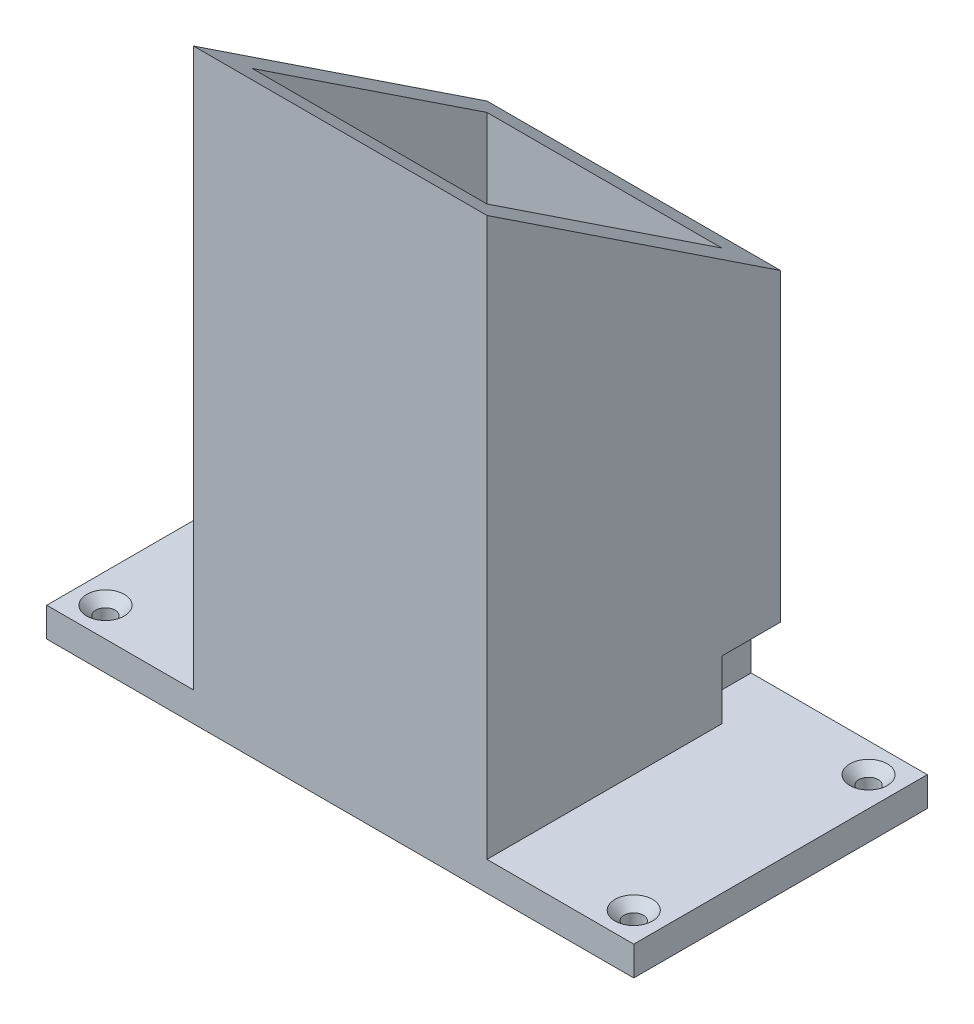
from build123d import *

# Parameters (mm, degrees)
SKETCH1_W                                            = 50
SKETCH1_H                                            = 10
SKETCH1_W_2                                          = 100
SKETCH1_H_2                                          = 200
BOSS_EXTRUDE1_DEPTH                                  = 100
CUT_EXTRUDE1_DEPTH                                   = 174.205080757
CUT_EXTRUDE1_DEPTH_BACK                              = 174.205080757
SKETCH7_W                                            = 80
SKETCH7_H                                            = 80
CUT_EXTRUDE2_DEPTH                                   = 100
SKETCH8_R                                            = 20
CUT_EXTRUDE3_DEPTH                                   = 20
CSK_FOR_M6_HEXAGON_LOBULAR_SOCKET_RAISED_D           = 6.6
CSK_FOR_M6_HEXAGON_LOBULAR_SOCKET_RAISED_CSINK_D     = 12.8
CSK_FOR_M6_HEXAGON_LOBULAR_SOCKET_RAISED_CSINK_ANGLE = 90
SKETCH13_W                                           = 20
SKETCH13_H                                           = 20
CUT_EXTRUDE4_DEPTH                                   = 10


with BuildPart() as part:
    # Sketch1 → Boss-Extrude1 (new body)
    with BuildSketch(Plane.XY):
        with Locations((-75, -95)):
            Rectangle(SKETCH1_W, SKETCH1_H)
        Rectangle(SKETCH1_W_2, SKETCH1_H_2)
        with Locations((75, -95)):
            Rectangle(SKETCH1_W, SKETCH1_H)
    extrude(amount=BOSS_EXTRUDE1_DEPTH)

    # Sketch5 → Cut-Extrude1 (cut, two sides: drawn at the far end of the back side and taken through both)
    with BuildSketch(Plane(origin=(0, 0, 0), x_dir=(0, 0, -1), z_dir=(1, 0, 0)).offset(-CUT_EXTRUDE1_DEPTH_BACK)):
        Polygon((-481.193494813, 352.459484715), (-100, 100), (0, 33.771302986), (381.193494813, -218.688181728), (886.112464242, 543.698807897), (23.725474617, 1114.84647434), align=None)
    extrude(amount=CUT_EXTRUDE1_DEPTH + CUT_EXTRUDE1_DEPTH_BACK, mode=Mode.SUBTRACT)

    # Sketch7 → Cut-Extrude2 (cut, symmetric)
    with BuildSketch(Plane(origin=(0, 0, 0), x_dir=(1, 0, 0), z_dir=(0, 1, 0))):
        with Locations((0, -50)):
            Rectangle(SKETCH7_W, SKETCH7_H)
    extrude(amount=CUT_EXTRUDE2_DEPTH, both=True, mode=Mode.SUBTRACT)

    # Sketch8 → Cut-Extrude3 (cut)
    with BuildSketch(Plane(origin=(0, 0, 0), x_dir=(-1, 0, 0), z_dir=(0, 0, -1))):
        with Locations((0, -40)):
            Circle(SKETCH8_R)
    extrude(amount=-CUT_EXTRUDE3_DEPTH, mode=Mode.SUBTRACT)

    # CSK for M6 Hexagon lobular socket raised CTSK head screws1 (through all)
    with Locations(Plane(origin=(0, -90, 0), x_dir=(1, 0, 0), z_dir=(0, 1, 0))):
        with Locations((-90, -10), (-90, -90), (90, -10), (90, -90)):
            CounterSinkHole(CSK_FOR_M6_HEXAGON_LOBULAR_SOCKET_RAISED_D / 2, CSK_FOR_M6_HEXAGON_LOBULAR_SOCKET_RAISED_CSINK_D / 2, counter_sink_angle=CSK_FOR_M6_HEXAGON_LOBULAR_SOCKET_RAISED_CSINK_ANGLE)

    # Sketch13 → Cut-Extrude4 (cut)
    with BuildSketch(Plane(origin=(50, 0, 0), x_dir=(0, 0, -1), z_dir=(1, 0, 0))):
        with Locations((-10, -80)):
            Rectangle(SKETCH13_W, SKETCH13_H)
    extrude(amount=-CUT_EXTRUDE4_DEPTH, mode=Mode.SUBTRACT)


solid = part.part
